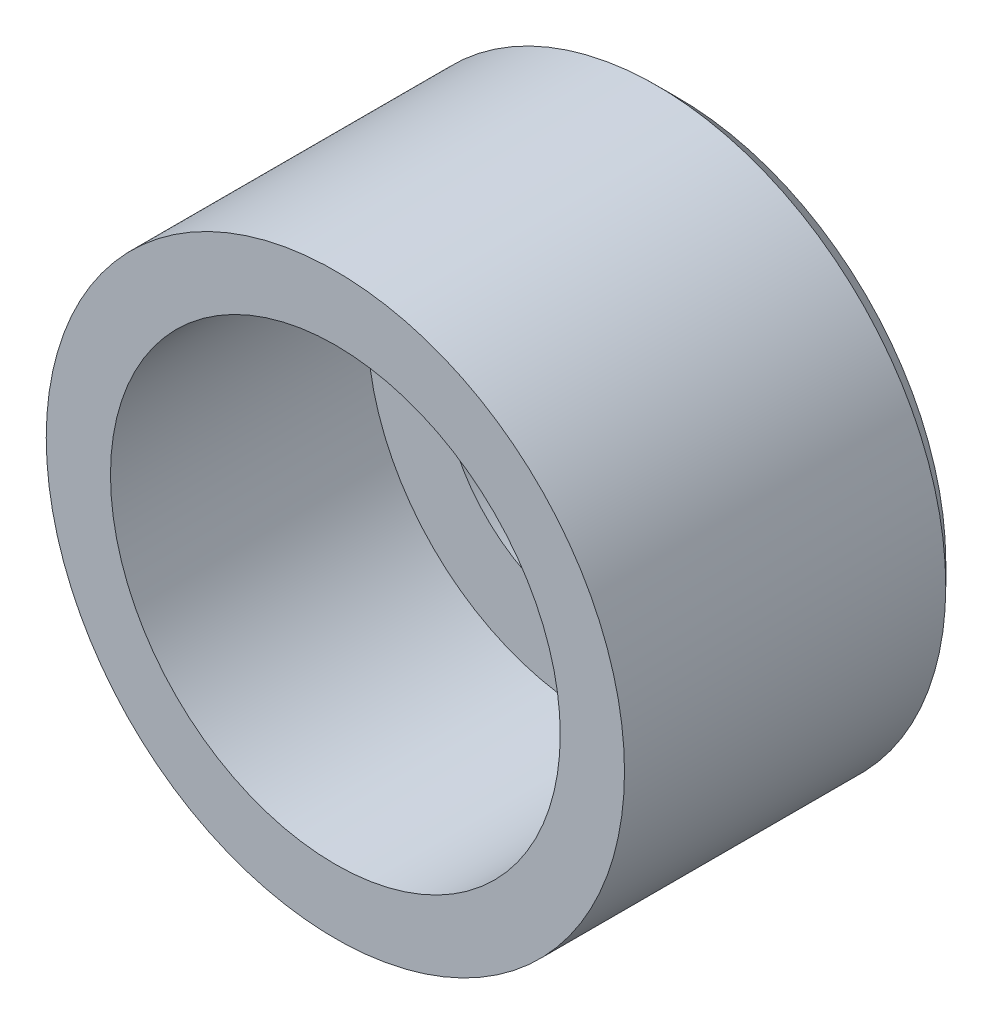
SolidWorks part; units mm, degrees
material "S45C"
ref_plane "Front Plane" through (0, 0, 0) normal (0, 0, 1) x (1, 0, 0)
ref_plane "Top Plane" through (0, 0, 0) normal (0, 1, 0) x (1, 0, 0)
ref_plane "Right Plane" through (0, 0, 0) normal (1, 0, 0) x (0, 0, -1)
sketch "Sketch1" plane through (0, 0, 0) normal (0, 0, 1) x (1, 0, 0)
  circle A0 centre (0, 0) radius 27
  circle A1 centre (0, 0) radius 14
  dimension "D1" = 54
  dimension "D2" = 28
extrude "Boss-Extrude1" add sketch "Sketch1" along normal blind 32
sketch "Sketch2" plane through (0, 0, 32) normal (0, 0, 1) x (1, 0, 0)
  circle A0 centre (0, 0) radius 21
  dimension "D1" = 42
extrude "Cut-Extrude1" cut sketch "Sketch2" against normal blind 24
chamfer "Chamfer1" distance 2 angle 45 1 edges at (27, 0, 0)
